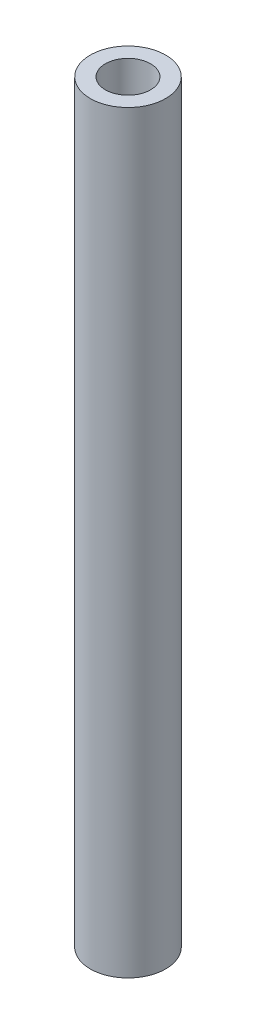
SolidWorks part; units mm, degrees
ref_plane "前视基准面" through (0, 0, 0) normal (0, 0, 1) x (1, 0, 0)
ref_plane "上视基准面" through (0, 0, 0) normal (0, 1, 0) x (1, 0, 0)
ref_plane "右视基准面" through (0, 0, 0) normal (1, 0, 0) x (0, 0, -1)
sketch "草图1" plane through (0, 0, 0) normal (0, 1, 0) x (1, 0, 0)
  circle A0 centre (0, 0) radius 3
  circle A1 centre (0, 0) radius 5
  dimension "D1" = 10
  dimension "D2" = 6
extrude "凸台-拉伸1" add sketch "草图1" along normal blind 100
